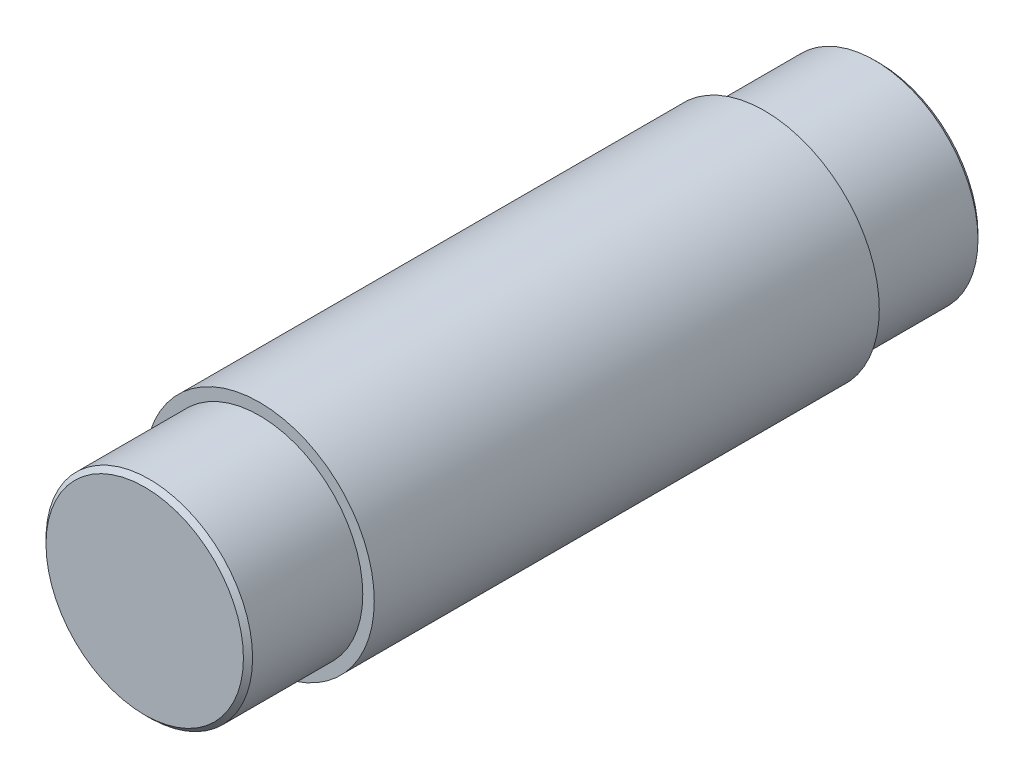
from build123d import *

# Parameters (mm, degrees)
SKETCH_1_R      = 25
EXTRUDE_1_DEPTH = 55
SKETCH_2_R      = 22.5
EXTRUDE_2_DEPTH = 25
EXTRUDE_START   = 25
SKETCH_3_R      = 22.5
EXTRUDE_3_DEPTH = 25
CHAMFER_1_SIZE  = 1


with BuildPart() as part:
    # 草图1 → 凸台-拉伸1 (new, symmetric)
    with BuildSketch(Plane.XY):
        Circle(SKETCH_1_R)
    extrude(amount=EXTRUDE_1_DEPTH, both=True)

    # 草图2 → 凸台-拉伸2 (add)
    with BuildSketch(Plane.XY.offset(55)):
        Circle(SKETCH_2_R)
    extrude(amount=EXTRUDE_2_DEPTH)

    # 草图3 → 凸台-拉伸3 (add)
    with BuildSketch(Plane(origin=(0, 0, -55), x_dir=(-1, 0, 0), z_dir=(0, 0, -1)).offset(EXTRUDE_START)):
        with Locations(Location((0, 0, 0), (0, 0, 180))):
            Circle(SKETCH_3_R)
    extrude(amount=-EXTRUDE_3_DEPTH)

    # 倒角1
    chamfer_1_edges = [part.edges().sort_by_distance(p)[0] for p in [
        (-22.5, 0, -80),
        (-22.5, 0, 80),
    ]]
    chamfer(chamfer_1_edges, length=CHAMFER_1_SIZE)


solid = part.part
